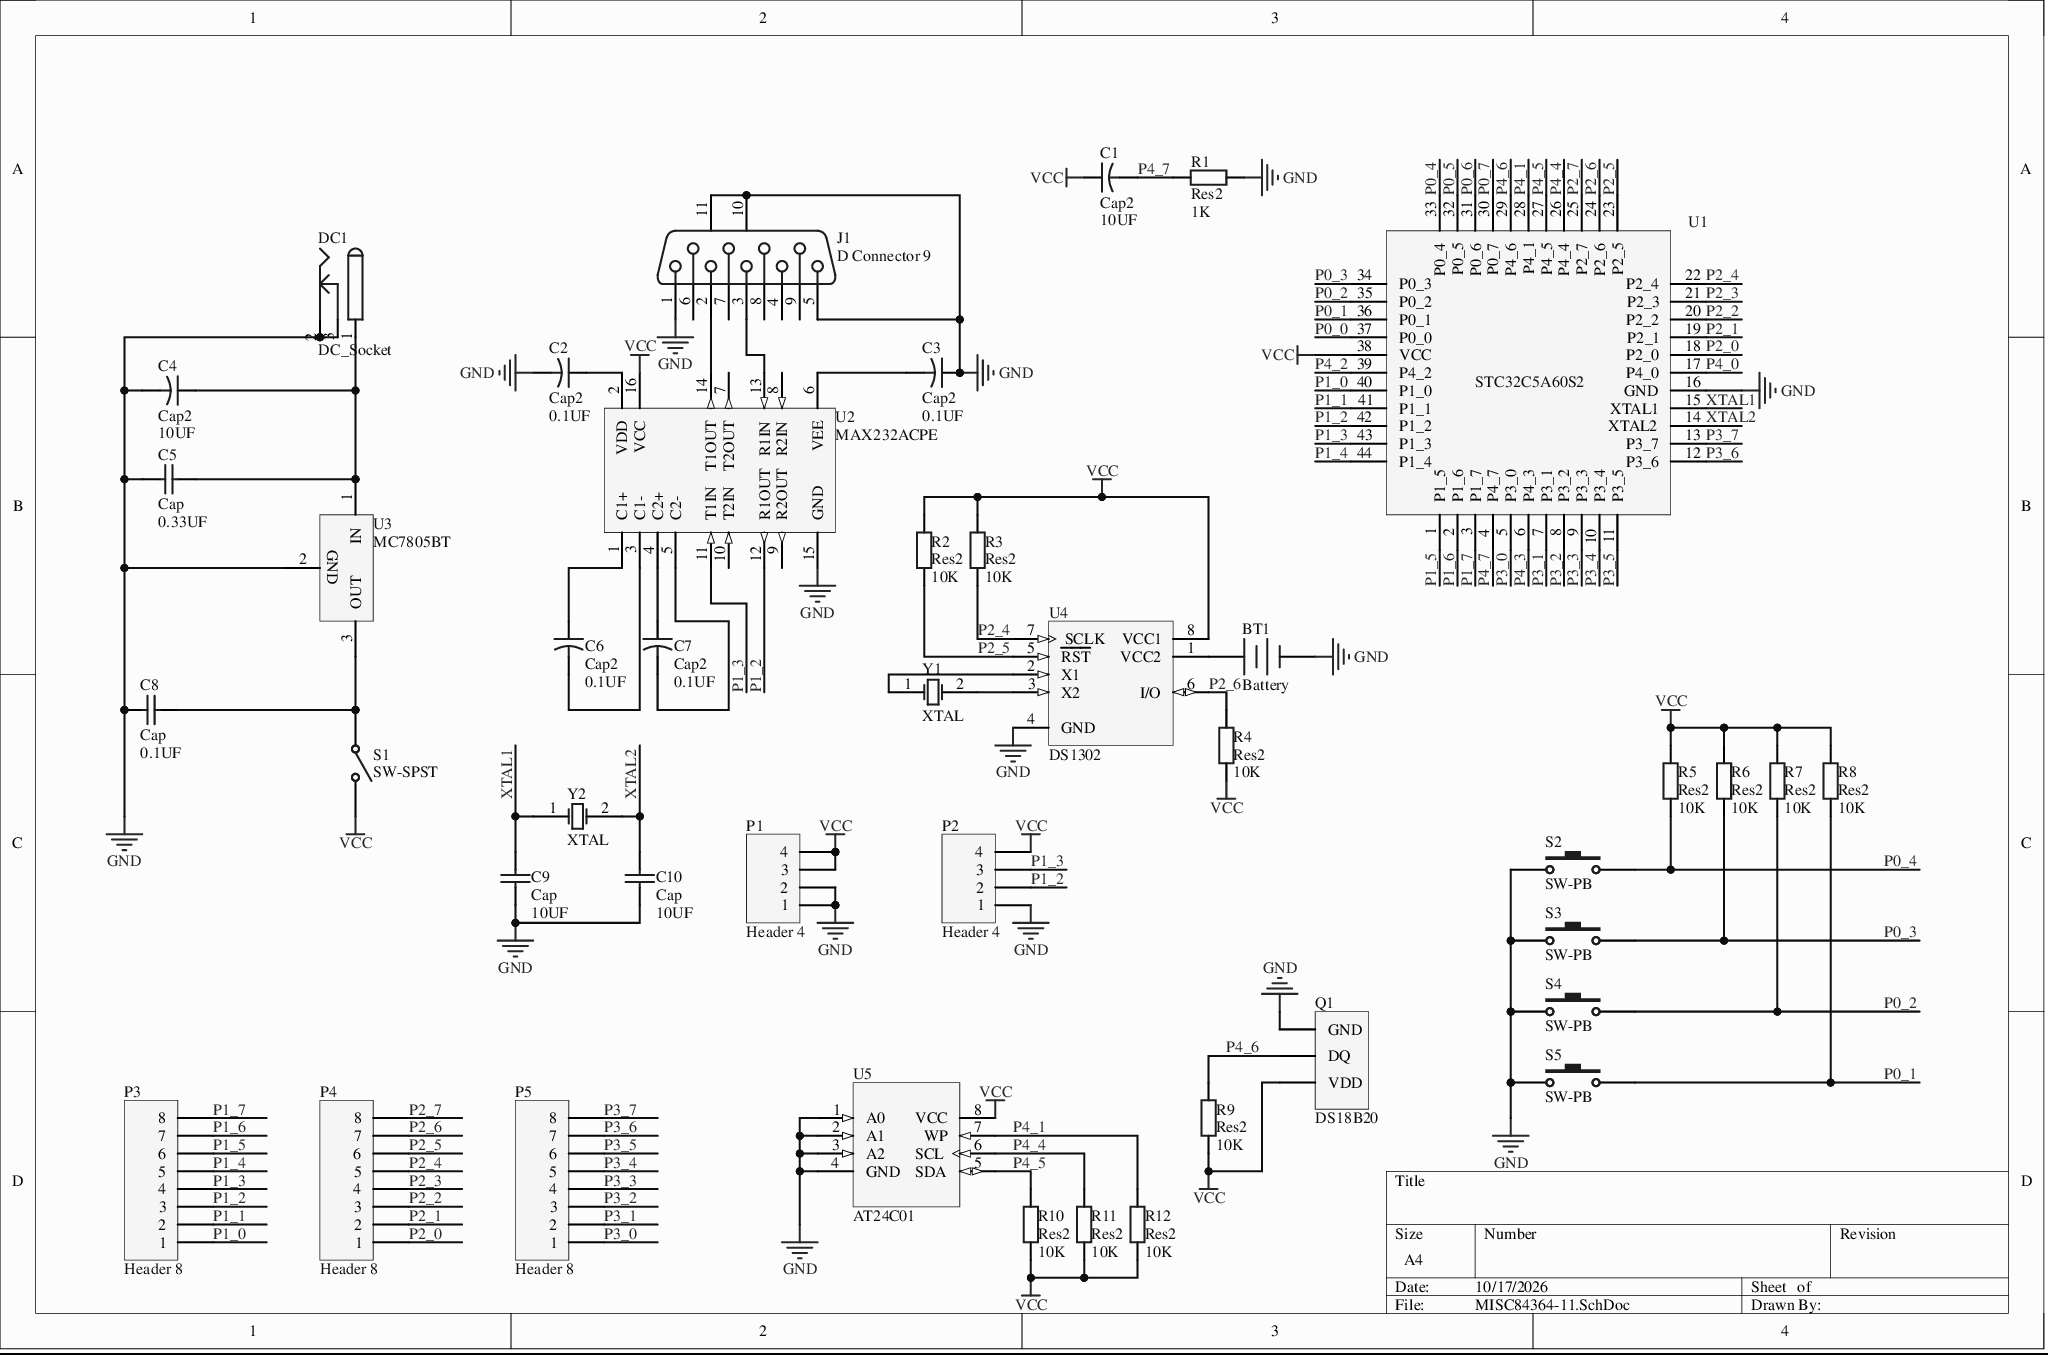
[diagram p0: MISC84364-11.SchDoc]
# Altium project MISC84364-3.PrjPcb
1 sheet, 43 parts. Net scope: global (net labels, ports and power ports of the same name join across sheets).
Board file: MISC84364.PcbDoc

## Sheet MISC84364-11.SchDoc
size A4

### Parts
BT1  Battery  [BAT-2]
C1  Cap2  value 10UF  [CAPR5-4X5]
C2  Cap2  value 0.1UF  [CAPR5-4X5]
C3  Cap2  value 0.1UF  [CAPR5-4X5]
C4  Cap2  value 10UF  [CAPR5-4X5]
C5  Cap  value 0.33UF  [RAD-0.1]
C6  Cap2  value 0.1UF  [CAPR5-4X5]
C7  Cap2  value 0.1UF  [CAPR5-4X5]
C8  Cap  value 0.1UF  [RAD-0.1]
C9  Cap  value 10UF  [RAD-0.1]
C10  Cap  value 10UF  [RAD-0.1]
DC1  DC_Socket  [DC-002]
J1  D Connector 9  [DSUB1.385-2H9]
P1  Header 4  [HDR1X4]
P2  Header 4  [HDR1X4]
P3  Header 8  [HDR1X8]
P4  Header 8  [HDR1X8]
P5  Header 8  [HDR1X8]
Q1  DS18B20  [HDR1X3]
R1  Res2  value 1K  [AXIAL-0.4]
R2  Res2  value 10K  [AXIAL-0.4]
R3  Res2  value 10K  [AXIAL-0.4]
R4  Res2  value 10K  [AXIAL-0.4]
R5  Res2  value 10K  [AXIAL-0.4]
R6  Res2  value 10K  [AXIAL-0.4]
R7  Res2  value 10K  [AXIAL-0.4]
R8  Res2  value 10K  [AXIAL-0.4]
R9  Res2  value 10K  [AXIAL-0.4]
R10  Res2  value 10K  [AXIAL-0.4]
R11  Res2  value 10K  [AXIAL-0.4]
R12  Res2  value 10K  [AXIAL-0.4]
S1  SW-SPST  [SPST-2]
S2  SW-PB  [SPST-2]
S3  SW-PB  [SPST-2]
S4  SW-PB  [SPST-2]
S5  SW-PB  [SPST-2]
U1  STC32C5A60S2  [LQFP48 7X7]
U2  MAX232ACPE  [PE16A]
U3  MC7805BT  [221A-04]
U4  DS1302  [DIP8]
U5  AT24C01  [DIP-8]
Y1  XTAL  [R38]
Y2  XTAL  [R38]

### Nets
GND: BT1.2(-) C2.2 C3.1 C4.2 C5.1 C8.1 C9.1 C10.1 DC1.2 DC1.3 J1.1 J1.5 J1.10(MH1) J1.11(MH2) P1.1 P1.2 P2.1 Q1.1(GND) R1.1 S2.1 S3.1 S4.1 S5.1 U1.16(GND) U2.15(GND) U3.2(GND) U4.4(GND) U5.1(A0) U5.2(A1) U5.3(A2) U5.4(GND)
VCC: C1.1 P1.3 P1.4 P2.4 Q1.3(VDD) R2.2 R3.2 R4.1 R5.2 R6.2 R7.2 R8.2 R9.1 R10.1 R11.1 R12.1 S1.2(NO) U1.38(VCC) U2.16(VCC) U4.8(VCC1) U5.8(VCC)
P0_0: U1.37(P0_0)
P0_1: R8.1 S5.2 U1.36(P0_1)
P0_2: R7.1 S4.2 U1.35(P0_2)
P0_3: R6.1 S3.2 U1.34(P0_3)
P0_4: R5.1 S2.2 U1.33(P0_4)
P0_5: U1.32(P0_5)
P0_6: U1.31(P0_6)
P0_7: U1.30(P0_7)
P1_0: P3.1 U1.40(P1_0)
P1_1: P3.2 U1.41(P1_1)
P1_2: P2.2 P3.3 U1.42(P1_2) U2.12(R1OUT)
P1_3: P2.3 P3.4 U1.43(P1_3) U2.11(T1IN)
P1_4: P3.5 U1.44(P1_4)
P1_5: P3.6 U1.1(P1_5)
P1_6: P3.7 U1.2(P1_6)
P1_7: P3.8 U1.3(P1_7)
P2_0: P4.1 U1.18(P2_0)
P2_1: P4.2 U1.19(P2_1)
P2_2: P4.3 U1.20(P2_2)
P2_3: P4.4 U1.21(P2_3)
P2_4: P4.5 R3.1 U1.22(P2_4) U4.7(SCLK)
P2_5: P4.6 R2.1 U1.23(P2_5) U4.5(~{RST})
P2_6: P4.7 R4.2 U1.24(P2_6) U4.6(I/O)
P2_7: P4.8 U1.25(P2_7)
P3_0: P5.1 U1.5(P3_0)
P3_1: P5.2 U1.7(P3_1)
P3_2: P5.3 U1.8(P3_2)
P3_3: P5.4 U1.9(P3_3)
P3_4: P5.5 U1.10(P3_4)
P3_5: P5.6 U1.11(P3_5)
P3_6: P5.7 U1.12(P3_6)
P3_7: P5.8 U1.13(P3_7)
P4_0: U1.17(P4_0)
P4_1: R12.2 U1.28(P4_1) U5.7(WP)
P4_2: U1.39(P4_2)
P4_3: U1.6(P4_3)
P4_4: R11.2 U1.26(P4_4) U5.6(SCL)
P4_5: R10.2 U1.27(P4_5) U5.5(SDA)
P4_6: Q1.2(DQ) R9.2 U1.29(P4_6)
P4_7: C1.2 R1.2 U1.4(P4_7)
XTAL1: C9.2 U1.15(XTAL1) Y2.1(OSC1)
XTAL2: C10.2 U1.14(XTAL2) Y2.2(OSC2)
NetBT1_1: BT1.1(+) U4.1(VCC2)
NetC2_1: C2.1 U2.2(VDD)
NetC3_2: C3.2 U2.6(VEE)
NetC4_1: C4.1 C5.2 DC1.1 U3.1(IN)
NetC6_1: C6.1 U2.1(C1+)
NetC6_2: C6.2 U2.3(C1-)
NetC7_1: C7.1 U2.4(C2+)
NetC7_2: C7.2 U2.5(C2-)
NetC8_2: C8.2 S1.1(COMMON) U3.3(OUT)
NetJ1_2: J1.2 U2.14(T1OUT)
NetJ1_3: J1.3 U2.13(R1IN)
NetU4_2: U4.2(X1) Y1.1(OSC1)
NetU4_3: U4.3(X2) Y1.2(OSC2)

Not connected (* = marked no-connect by the designer): J1 4 6 7 8 9; U2 7(T2OUT) 8(R2IN) 9(R2OUT) 10(T2IN)

### Library data of the parts
BT1 = Battery: Multicell Battery; Published: 24-Mar-1999; LatestRevisionDate: 17-Jul-2002; LatestRevisionNote: Re-released for DXP Platform.; PackageReference: BAT-2; PackageDescription: Battery; 2 Leads; Publisher: Altium Limited
C1-C4 C6 C7 = Cap2: Capacitor; Published: 23-Sep-2002; PackageReference: CAPR5-4X5; PackageDescription: Capacitor; 2 Leads; Publisher: Altium Limited
C5 C8-C10 = Cap: Capacitor; Published: 8-Jun-2000; LatestRevisionDate: 17-Jul-2002; LatestRevisionNote: Re-released for DXP Platform.; PackageReference: RAD-0.3; PackageDescription: Radial Cap, Thru-Hole; 2 Leads; 0.3 in Pin Spacing; Publisher: Altium Limited
J1 = D Connector 9: Receptacle Assembly, 9 Position, Right Angle; PackageDocument: O; Positions: 9; Published: 15-Jun-2001; LatestRevisionDate: 17-Jul-2002; LatestRevisionNote: Re-released for DXP Platform.; DatasheetDocument: 1-Sep-1999; PackageReference: 788750; Orientation: Right Angle; Gender: Receptacle; Publisher: Altium Limited
P1 P2 = Header 4: Header, 4-Pin; LatestRevisionDate: 17-Jul-2002; LatestRevisionNote: Re-released for DXP Platform.; Publisher: Altium Limited
P3-P5 = Header 8: Header, 8-Pin; LatestRevisionDate: 17-Jul-2002; LatestRevisionNote: Re-released for DXP Platform.; Publisher: Altium Limited
Q1 = DS18B20: 数字温度计; BOM名称: parameter BOM name text digital thermometer
R1-R12 = Res2: Resistor; Published: 8-Jun-2000; LatestRevisionDate: 17-Jul-2002; LatestRevisionNote: Re-released for DXP Platform.; PackageReference: AXIAL-0.4; PackageDescription: Axial Device, Thru-Hole; 2 Leads; 0.4 in Pin Spacing; Publisher: Altium Limited
S1 = SW-SPST: Single-Pole, Single-Throw Switch; Published: 24-Mar-1999; LatestRevisionDate: 17-Jul-2002; LatestRevisionNote: Re-released for DXP Platform.; PackageReference: SPST-2; PackageDescription: Switch; 2 Leads; Publisher: Altium Limited
S2-S5 = SW-PB: Switch; Published: 24-Mar-1999; LatestRevisionDate: 17-Jul-2002; LatestRevisionNote: Re-released for DXP Platform.; PackageReference: SPST-2; PackageDescription: Switch; 2 Leads; Publisher: Altium Limited
U2 = MAX232ACPE: +5V Powered, Multi-Channel RS-232 Driver/Receiver; Package Information: Latest Revision: 1997; Code - JEDEC: MS-001-BB; Published: 16-Jan-2001; Revision: 17-Jul-2002: Re-released for DXP Platform.; Package Reference: PE16A; Publisher: Altium Limited
U3 = MC7805BT: 3-Terminal Positive Fixed Voltage Regulator; Note: Pin 2 is electrically connected to TAB; Code - JEDEC: TO-262-AA; Published: 17-Jul-2002; Datasheet: Linear and Interface Integrated Circuits, DL128 Rev2 (1988); Package Reference: 221A-04; Publisher: Altium Limited
U4 = DS1302: Trickle Charge Timekeeping Chip; Package Information: Latest Revision: 1999; Published: 13-Oct-2000; Revision: 17-Jul-2002: Re-released for DXP Platform.; Datasheet: Latest Revision: 2-Jul-1999; Package Reference: DIP8; Publisher: Altium Limited
U5 = AT24C01BN-SP25-T: 1Kbit (128 x 8), 2-wire Bus Automotive Serial EEPROM with Write Protect, 2.5V, 8-Pin SOIC, Tape & Reel; Published: 20-Sep-2010; DatasheetVersion: 8517C,  Jan-2009; PackageVersion: revC, Mar-2005; PackageReference: 8S1; PackageDescription: 8-Lead (0.150" Wide Body), Plastic Gull Wing Small Outline (JEDEC SOIC); Code_JEDEC: MS-012-AA; Code_IPC: SOIC127P600-8; ComponentLink1Description: Manufacturer Link; ComponentLink2Description: Datasheet; ComponentLink2URL: example.com/doc8517.pdf; ComponentLink3Description: Atmel.com Home; Publisher: Altium Limited
Y1 Y2 = XTAL: Crystal Oscillator; Published: 8-Jun-2000; LatestRevisionDate: 17-Jul-2002; LatestRevisionNote: Re-released for DXP Platform.; PackageReference: R38; PackageDescription: Crystal, Thru-Hole; 2 Leads; Body 3.1 x 8.2 mm (Dia.xH); Publisher: Altium Limited